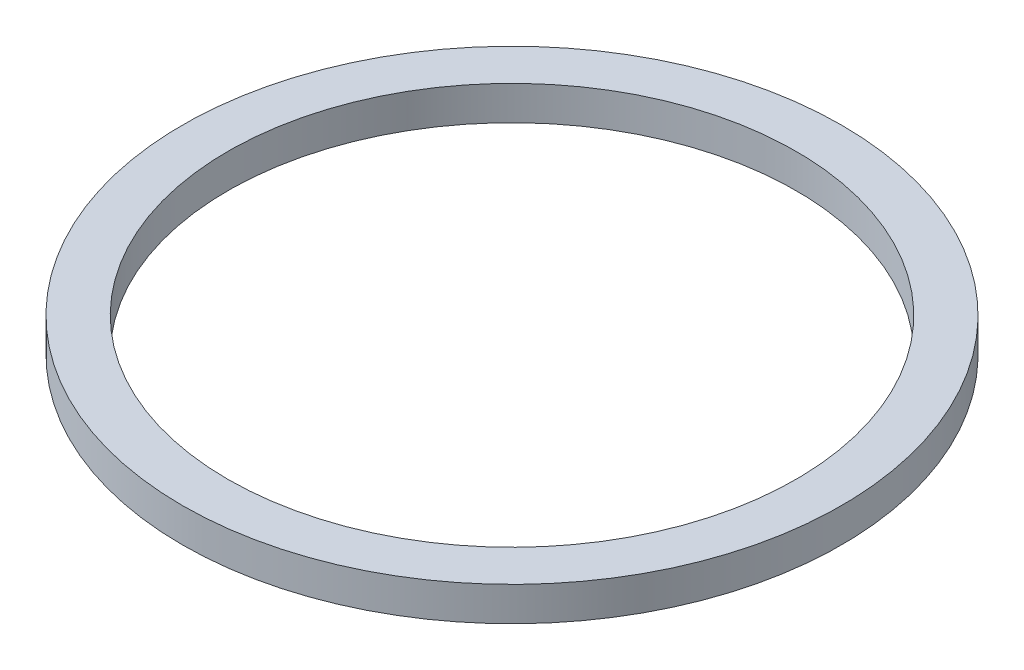
SolidWorks part; units mm, degrees
material "哈碳纤"
ref_plane "前视基准面" through (0, 0, 0) normal (0, 0, 1) x (1, 0, 0)
ref_plane "上视基准面" through (0, 0, 0) normal (0, 1, 0) x (1, 0, 0)
ref_plane "右视基准面" through (0, 0, 0) normal (1, 0, 0) x (0, 0, -1)
other "Configuration Table"
sketch "草图1" plane through (0, 0, 0) normal (0, 1, 0) x (1, 0, 0)
  circle A0 centre (0, 0) radius 29
  circle A1 centre (0, 0) radius 25
  dimension "D1" = 58
  dimension "D2" = 50
extrude "凸台-拉伸1" add sketch "草图1" along normal blind 3
